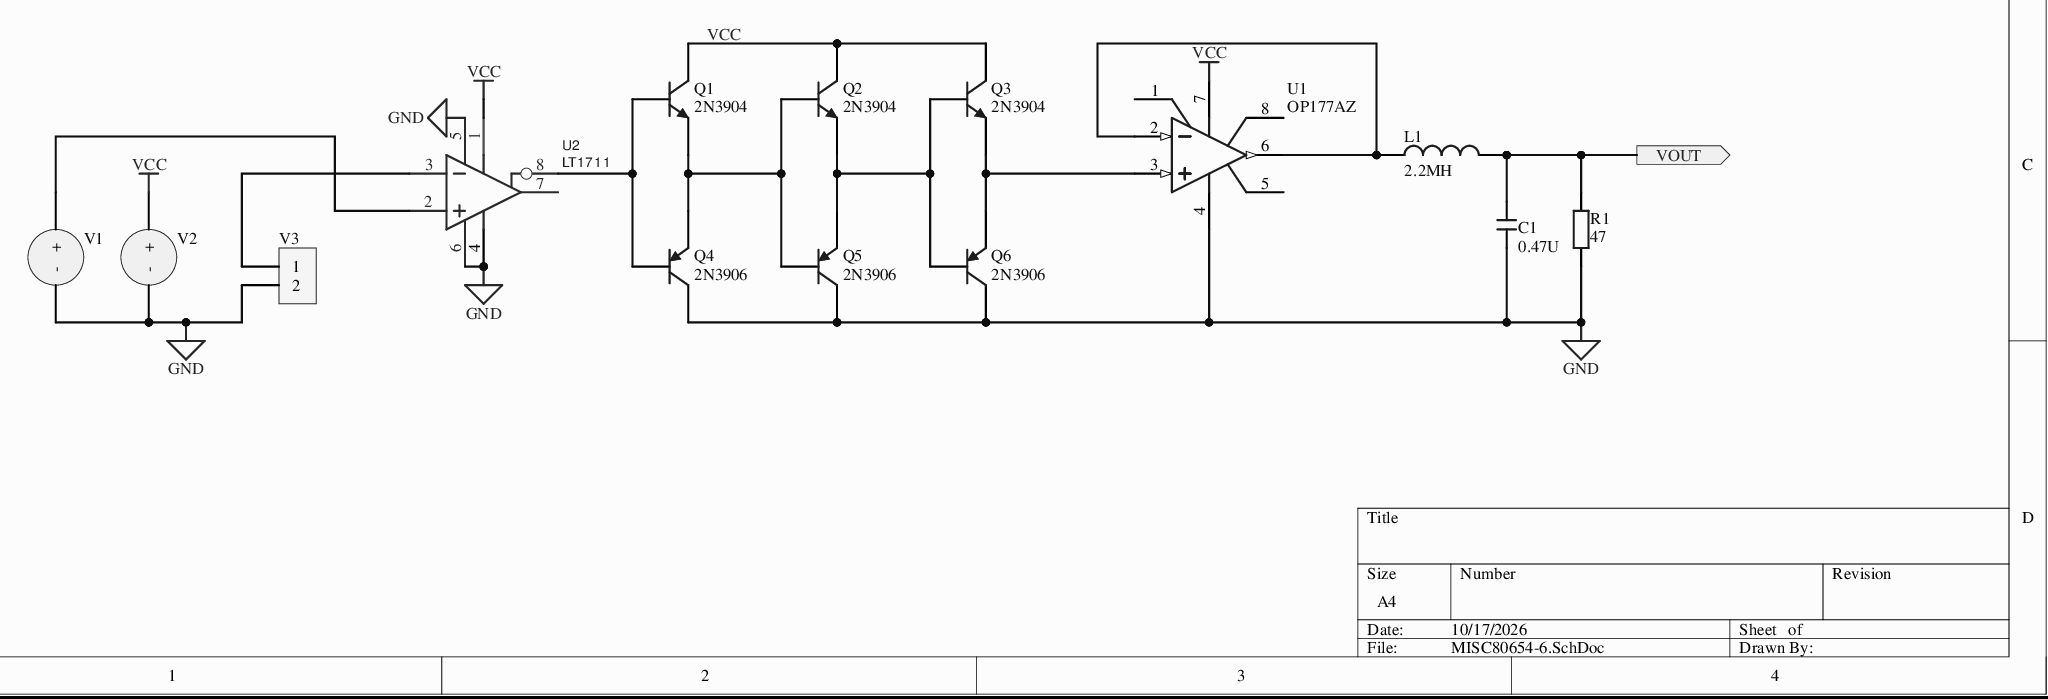
[diagram p0: MISC80654-6.SchDoc]
# Altium project MISC80654-2.PrjPcb
1 sheet, 14 parts. Net scope: flat (ports and power ports of the same name join across sheets).
Board file: MISC80654.PcbDoc

## Sheet MISC80654-6.SchDoc
size A4

### Parts
C1  0.47U  [CC 1.8*3.6]
L1  2.2MH  [AL0307]
Q1  2N3904  [TO-92A]
Q2  2N3904  [TO-92A]
Q3  2N3904  [TO-92A]
Q4  2N3906  [TO-92A]
Q5  2N3906  [TO-92A]
Q6  2N3906  [TO-92A]
R1  47  [RS 1/4W]
U1  OP177AZ  [Q-8]
U2  LT1711  [SOP8]
V1  Current source  [Fe-HDR1X2/2.54-S]  (value not drawn)
V2  Current source  [Fe-HDR1X2/2.54-S]  (value not drawn)
V3  Female HDR1X2  [Fe-HDR1X2/2.54-S]  (value not drawn)

### Ports
VOUT (out)

### Nets
GND: C1.2 Q4.3(C) Q5.3(C) Q6.3(C) R1.1 U1.4(V-) U2.4(V-) U2.5(LATCH_ENABLE) U2.6(GND) V1.2(-) V2.2(-) V3.2
VCC: Q1.3(C) Q2.3(C) Q3.3(C) U1.7(V+) U2.1(V+) V2.1(+)
NetC1_1: C1.1 L1.2 R1.2 ; port VOUT
NetL1_1: L1.1 U1.2(IN-) U1.6(OUT)
NetQ1_1: Q1.1(E) Q2.2(B) Q4.1(E) Q5.2(B)
NetQ1_2: Q1.2(B) Q4.2(B) U2.8(Q#_OUT)
NetQ2_1: Q2.1(E) Q3.2(B) Q5.1(E) Q6.2(B)
NetQ3_1: Q3.1(E) Q6.1(E) U1.3(IN+)
NetU2_2: U2.2(+IN) V1.1(+)
NetU2_3: U2.3(-IN) V3.1

Not connected (* = marked no-connect by the designer): U1 1(VOSTRIM)* 5(NC)* 8(VOSTRIM)*; U2 7(Q_OUT)*

### Library data of the parts
C1 = CC: Ceramic disc capacitor; BOM名称: Through-hole ceramic capacitor
L1 = L-AL: Color-band inductor; BOM名称: Color-band inductor
Q1-Q3 = 2N3904: NPN General Purpose Amplifier; Published: 8-Jun-2000; LatestRevisionDate: 15-Jan-2003; LatestRevisionNote: PCB Footprint 'BCY-W3/D4.7' replaced; DatasheetVersion: 1997; PackageVersion: Sep-1998; PackageReference: TO-92A; PackageDescription: TO, Flat Index; 3 In-Line, Axial Leads; Body Dia. 4.5mm; Leads 0.51 x 0.48 mm (max); ComponentLink1Description: Manufacturer Link; ComponentLink1URL: http://www.fairchildsemi.com/; ComponentLink2Description: Datasheet; ComponentLink2URL: http://www.fairchildsemi.com/ds/2N%2F2N3904.pdf; Publisher: Altium Limited
Q4-Q6 = 2N3906: PNP General Purpose Amplifier; Published: 8-Jun-2000; LatestRevisionDate: 15-Jan-2003; LatestRevisionNote: PCB Footprint 'BCY-W3/D4.7' replaced; DatasheetVersion: 1997; PackageVersion: Sep-1998; PackageReference: TO-92A; PackageDescription: TO, Flat Index; 3 In-Line, Axial Leads; Body Dia. 4.5mm; Leads 0.51 x 0.48 mm (max); ComponentLink1Description: Manufacturer Link; ComponentLink1URL: http://www.fairchildsemi.com/; ComponentLink2Description: Datasheet; ComponentLink2URL: http://www.fairchildsemi.com/ds/2N%2F2N3906.pdf; Publisher: Altium Limited
R1 = R-S: Color-band resistor; BOM名称: Color-band resistor
U1 = OP177AZ: Ultraprecision Operational Amplifier; Revision 1: 10-Jul-2000: SIM Model Added.; Revision 2: 17-Jul-2002: Re-released for DXP Platform.; Package Information: Latest Revision: 1998; Note: Pin 5 is not connected.; Published: 8-Jun-2000; Datasheet: Designer's Reference Manual CD (REV. B 1995); Package Reference: Q-8; Publisher: Altium Limited
U2 = LT1711CMS8#PBF
V1 V2 = 电流源